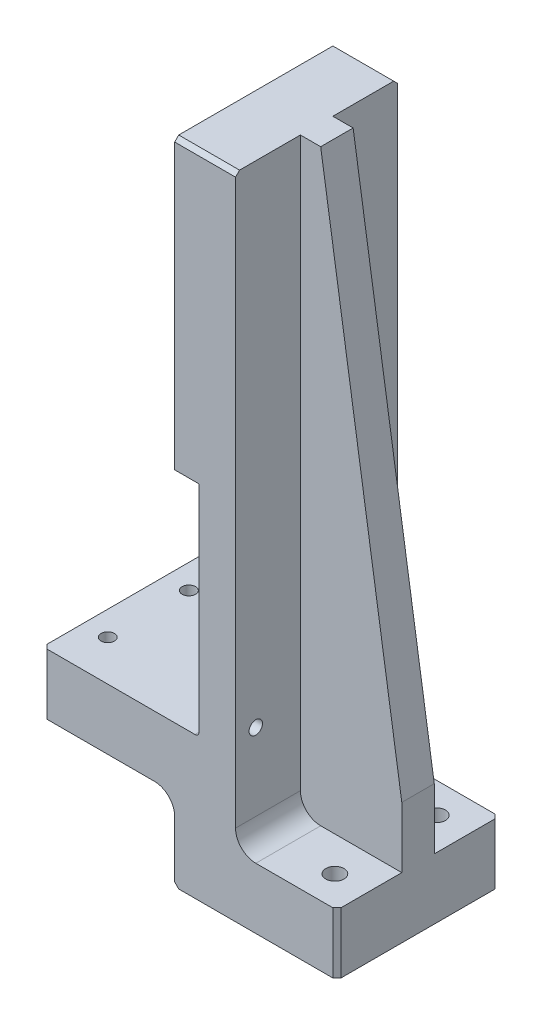
SolidWorks part; units mm, degrees
ref_plane "Front Plane" through (0, 0, 0) normal (0, 0, 1) x (1, 0, 0)
ref_plane "Top Plane" through (0, 0, 0) normal (0, 1, 0) x (1, 0, 0)
ref_plane "Right Plane" through (0, 0, 0) normal (1, 0, 0) x (0, 0, -1)
sketch "Sketch1" plane through (0, 0, 0) normal (0, 0, 1) x (1, 0, 0)
  line L0 (0, 0) -> (32.5, 0)
  line L1 (32.5, 0) -> (32.5, 125)
  line L2 (32.5, 125) -> (47.5, 125)
  line L3 (47.5, 125) -> (47.5, -20)
  line L4 (47.5, -20) -> (72.5, -20)
  line L5 (72.5, -20) -> (72.5, -35)
  line L6 (72.5, -35) -> (32.5, -35)
  line L7 (0, -15) -> (0, 0)
  line L8 (0, -15) -> (32.5, -15)
  line L9 (32.5, -15) -> (32.5, -35)
  dimension "D1" = 32.5
  dimension "D2" = 15
  dimension "D3" = 25
  dimension "D4" = 160
  dimension "D5" = 35
  dimension "D6" = 15
  dimension "D7" = 15
extrude "Boss-Extrude1" add sketch "Sketch1" along normal mid plane 40
sketch "Sketch2" plane through (0, 0, 0) normal (0, 0, 1) x (1, 0, 0)
  line L0 (47.5, 125) -> (52.5, 125)
  line L1 (52.5, 125) -> (72.5, -5)
  line L2 (72.5, -5) -> (72.5, -20)
  line L3 (72.5, -20) -> (47.5, -20)
  line L4 (47.5, -20) -> (47.5, 125)
  dimension "D1" = 5
  dimension "D2" = 15
extrude "Boss-Extrude2" add sketch "Sketch2" along normal mid plane 8
sketch "Sketch3" plane through (0, -20, 0) normal (0, 1, 0) x (1, 0, 0)
  line L1 (72.5, -20) -> (72.5, -4) construction
  circle A0 centre (64.5, -12.5) radius 2.25
  circle A1 centre (64.5, 12.5) radius 2.25
  dimension "D1" = 25
  dimension "D2" = 8
  dimension "D3" = 4.5
  dimension "D4" = 12.5
extrude "Cut-Extrude2" cut sketch "Sketch3" against normal through all
hole_wizard "M4 Tapped Hole1" positions "Sketch5" profile "Sketch4" tap size "M4" standard "Gb" end condition through all
sketch "Sketch5" plane through (0, 0, 0) normal (0, 1, 0) x (-1, 0, 0)
  line L0 (-6, -10) -> (-6, 10) construction
  line L3 (-6, 0) -> (0, 0) construction
  line L5 (0, 20) -> (0, -20) construction
  point P0 (-6, -10)
  point P1 (-6, 10)
  dimension "D1" = 20
  dimension "D2" = 6
cosmetic thread "Cosmetic Thread1" parameters "D2"=4
cosmetic thread "Cosmetic Thread2" parameters "D2"=4
sketch "Sketch4" plane through (6, 0, -10) normal (1, 0, 0) x (0, 0, 1)
  line L0 (0, 0) -> (0, 35)
  line L1 (0, 35) -> (1.65, 35)
  line L2 (1.65, 35) -> (1.65, 0)
  line L5 (1.65, 0) -> (0, 0)
  line L11 (0, -6.35) -> (0, 107.95) construction
  dimension "通孔螺纹孔钻头直径" = 3.3
  dimension "通孔螺纹孔钻头深度" = 35
hole_wizard "M4 Tapped Hole2" positions "Sketch9" profile "Sketch8" tap size "M4" standard "GB"
sketch "Sketch9" plane through (32.5, -167.0502, 16.0875) normal (-1, 0, 0) x (0, 0, 1)
  line L0 (-16.0875, 292.0502) -> (-16.0875, 251.0502) construction
  line L3 (3.9125, 292.0502) -> (-36.0875, 292.0502) construction
  point P0 (-16.0875, 276.0502)
  point P1 (-16.0875, 251.0502)
  dimension "D1" = 16
  dimension "D2" = 25
sketch "Sketch8" plane through (32.5, 109, 0) normal (0, 1, 0) x (0, 0, 1)
  line L0 (0, 0) -> (0, 12.4914)
  line L1 (0, 12.4914) -> (1.65, 11.5)
  line L2 (1.65, 11.5) -> (1.65, 0)
  line L5 (1.65, 0) -> (0, 0)
  line L10 (0, 12.4914) -> (-1.65, 11.5) construction
  line L11 (0, -6.35) -> (0, 107.95) construction
  dimension "螺纹孔钻头直径" = 3.3
  dimension "螺纹孔钻头深度" = 11.5
  dimension "导头角度" = 118
cosmetic thread "Cosmetic Thread6" parameters "D1"=8, "D2"=4
cosmetic thread "Cosmetic Thread7" parameters "D1"=8, "D2"=4
sketch "Sketch12" plane through (0, 0, -20) normal (0, 0, -1) x (-1, 0, 0)
  line L1 (-32.5, 0) -> (-38.5, 0)
  line L2 (-32.5, 0) -> (-32.5, 54)
  line L3 (-32.5, 54) -> (-38.5, 54)
  line L4 (-38.5, 0) -> (-38.5, 54)
  dimension "D1" = 6
  dimension "D2" = 54
extrude "Cut-Extrude3" cut sketch "Sketch12" against normal up to next
hole_wizard "M4 Tapped Hole3" positions "Sketch16" profile "Sketch15" tap size "M4" standard "Gb"
sketch "Sketch16" plane through (38.5, 0, 0) normal (-1, 0, 0) x (0, 0, 1)
  line L0 (20, 0) -> (-20, 0) construction
  point P0 (-15, 4)
  point P2 (15, 4)
  dimension "D1" = 30
  dimension "D2" = 15
  dimension "D3" = 4
sketch "Sketch15" plane through (38.5, 4, -15) normal (0, 1, 0) x (0, 0, 1)
  line L0 (0, 0) -> (0, 12.4914)
  line L1 (0, 12.4914) -> (1.65, 11.5)
  line L2 (1.65, 11.5) -> (1.65, 0)
  line L5 (1.65, 0) -> (0, 0)
  line L10 (0, 12.4914) -> (-1.65, 11.5) construction
  line L11 (0, -6.35) -> (0, 107.95) construction
  dimension "螺纹孔钻头直径" = 3.3
  dimension "螺纹孔钻头深度" = 11.5
  dimension "导头角度" = 118
cosmetic thread "Cosmetic Thread9" parameters "D1"=8, "D2"=4
cosmetic thread "Cosmetic Thread10" parameters "D1"=8, "D2"=4
chamfer "Chamfer1" distance 1 angle 45 7 edges at (40, 125, -20) (40, 125, 20) (72.5, -27.5, -20) (72.5, -27.5, 20) (0, -7.5, -20) (0, -7.5, 20) (32.5, -35, 0)
fillet "Fillet1" radius 1 1 edges at (38.5, 0, 0)
fillet "Fillet2" radius 5 3 edges at (32.5, -15, 0) (47.5, -20, 12) (47.5, -20, -12)
